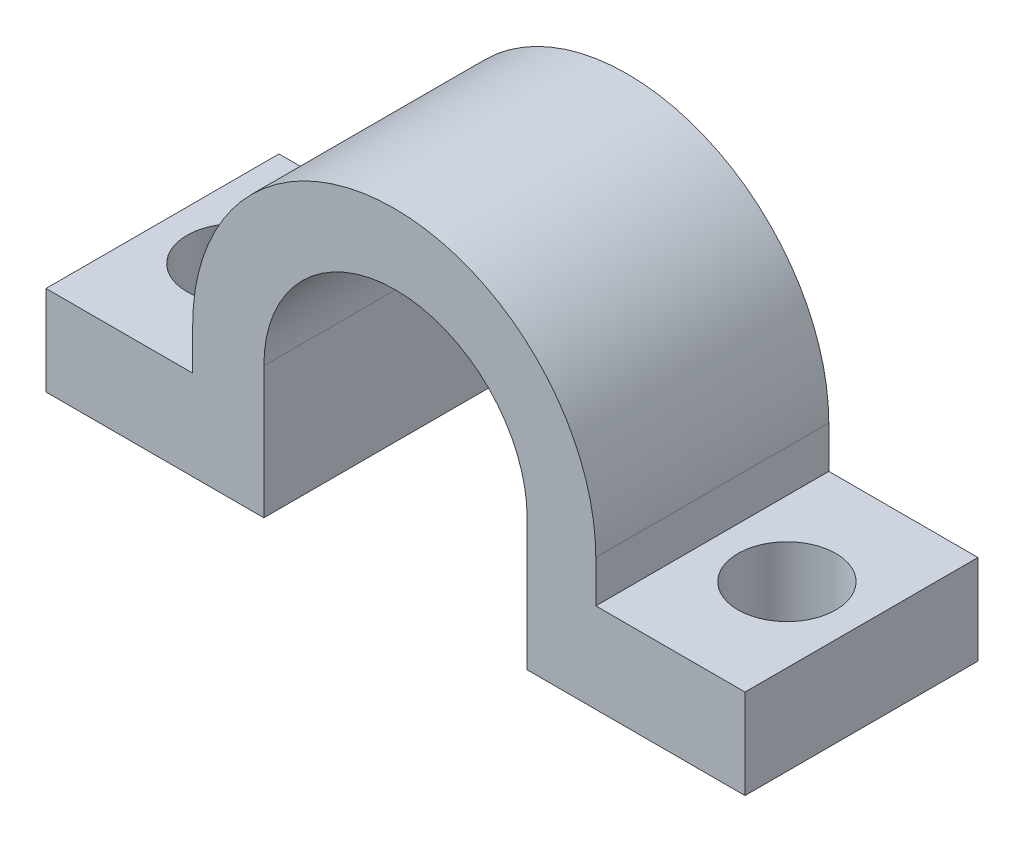
from build123d import *

# Parameters (mm, degrees)
EXTRUDE_1_DEPTH     = 10
SKETCH_2_R          = 2.1
CUT_EXTRUDE_1_DEPTH = 17.7


with BuildPart() as part:
    # 草图1 → 凸台-拉伸1 (new body)
    with BuildSketch(Plane.XY):
        with BuildLine():
            Line((-5.596661991, 5.185089456), (-5.596661991, 6.985089456))
            ThreePointArc((-5.596661991, 6.985089456), (0.053338009, 12.635089456), (5.703338009, 6.985089456))
            Line((5.703338009, 6.985089456), (5.703338009, 5.185089456))
            Line((5.703338009, 5.185089456), (5.703338009, 1.335089456))
            Line((5.703338009, 1.335089456), (15.053338009, 1.335089456))
            Line((15.053338009, 1.335089456), (15.053338009, 5.185089456))
            Line((15.053338009, 5.185089456), (8.65, 5.185089456))
            Line((8.65, 5.185089456), (8.65, 6.985089456))
            ThreePointArc((8.65, 6.985089456), (0, 15.635089456), (-8.65, 6.985089456))
            Line((-8.65, 6.985089456), (-8.65, 5.185089456))
            Line((-8.65, 5.185089456), (-14.946661991, 5.185089456))
            Line((-14.946661991, 5.185089456), (-14.946661991, 1.335089456))
            Line((-14.946661991, 1.335089456), (-5.596661991, 1.335089456))
            Line((-5.596661991, 1.335089456), (-5.596661991, 5.185089456))
        make_face()
    extrude(amount=EXTRUDE_1_DEPTH)

    # 草图2 → 切除-拉伸1 (cut)
    with BuildSketch(Plane(origin=(-970.090594905, 5.185089456, 1019.250263045), x_dir=(0, 0, 1), z_dir=(0, 1, 0))):
        with Locations((-1055.250263055, 981.942263912)):
            Circle(SKETCH_2_R)
        with Locations((-1055.250263055, 958.292263912)):
            Circle(SKETCH_2_R)
        with Locations((-1014.250263055, 958.292263912)):
            Circle(SKETCH_2_R)
        with Locations((-1014.250263055, 981.942263912)):
            Circle(SKETCH_2_R)
    extrude(amount=-CUT_EXTRUDE_1_DEPTH, mode=Mode.SUBTRACT)


solid = part.part
